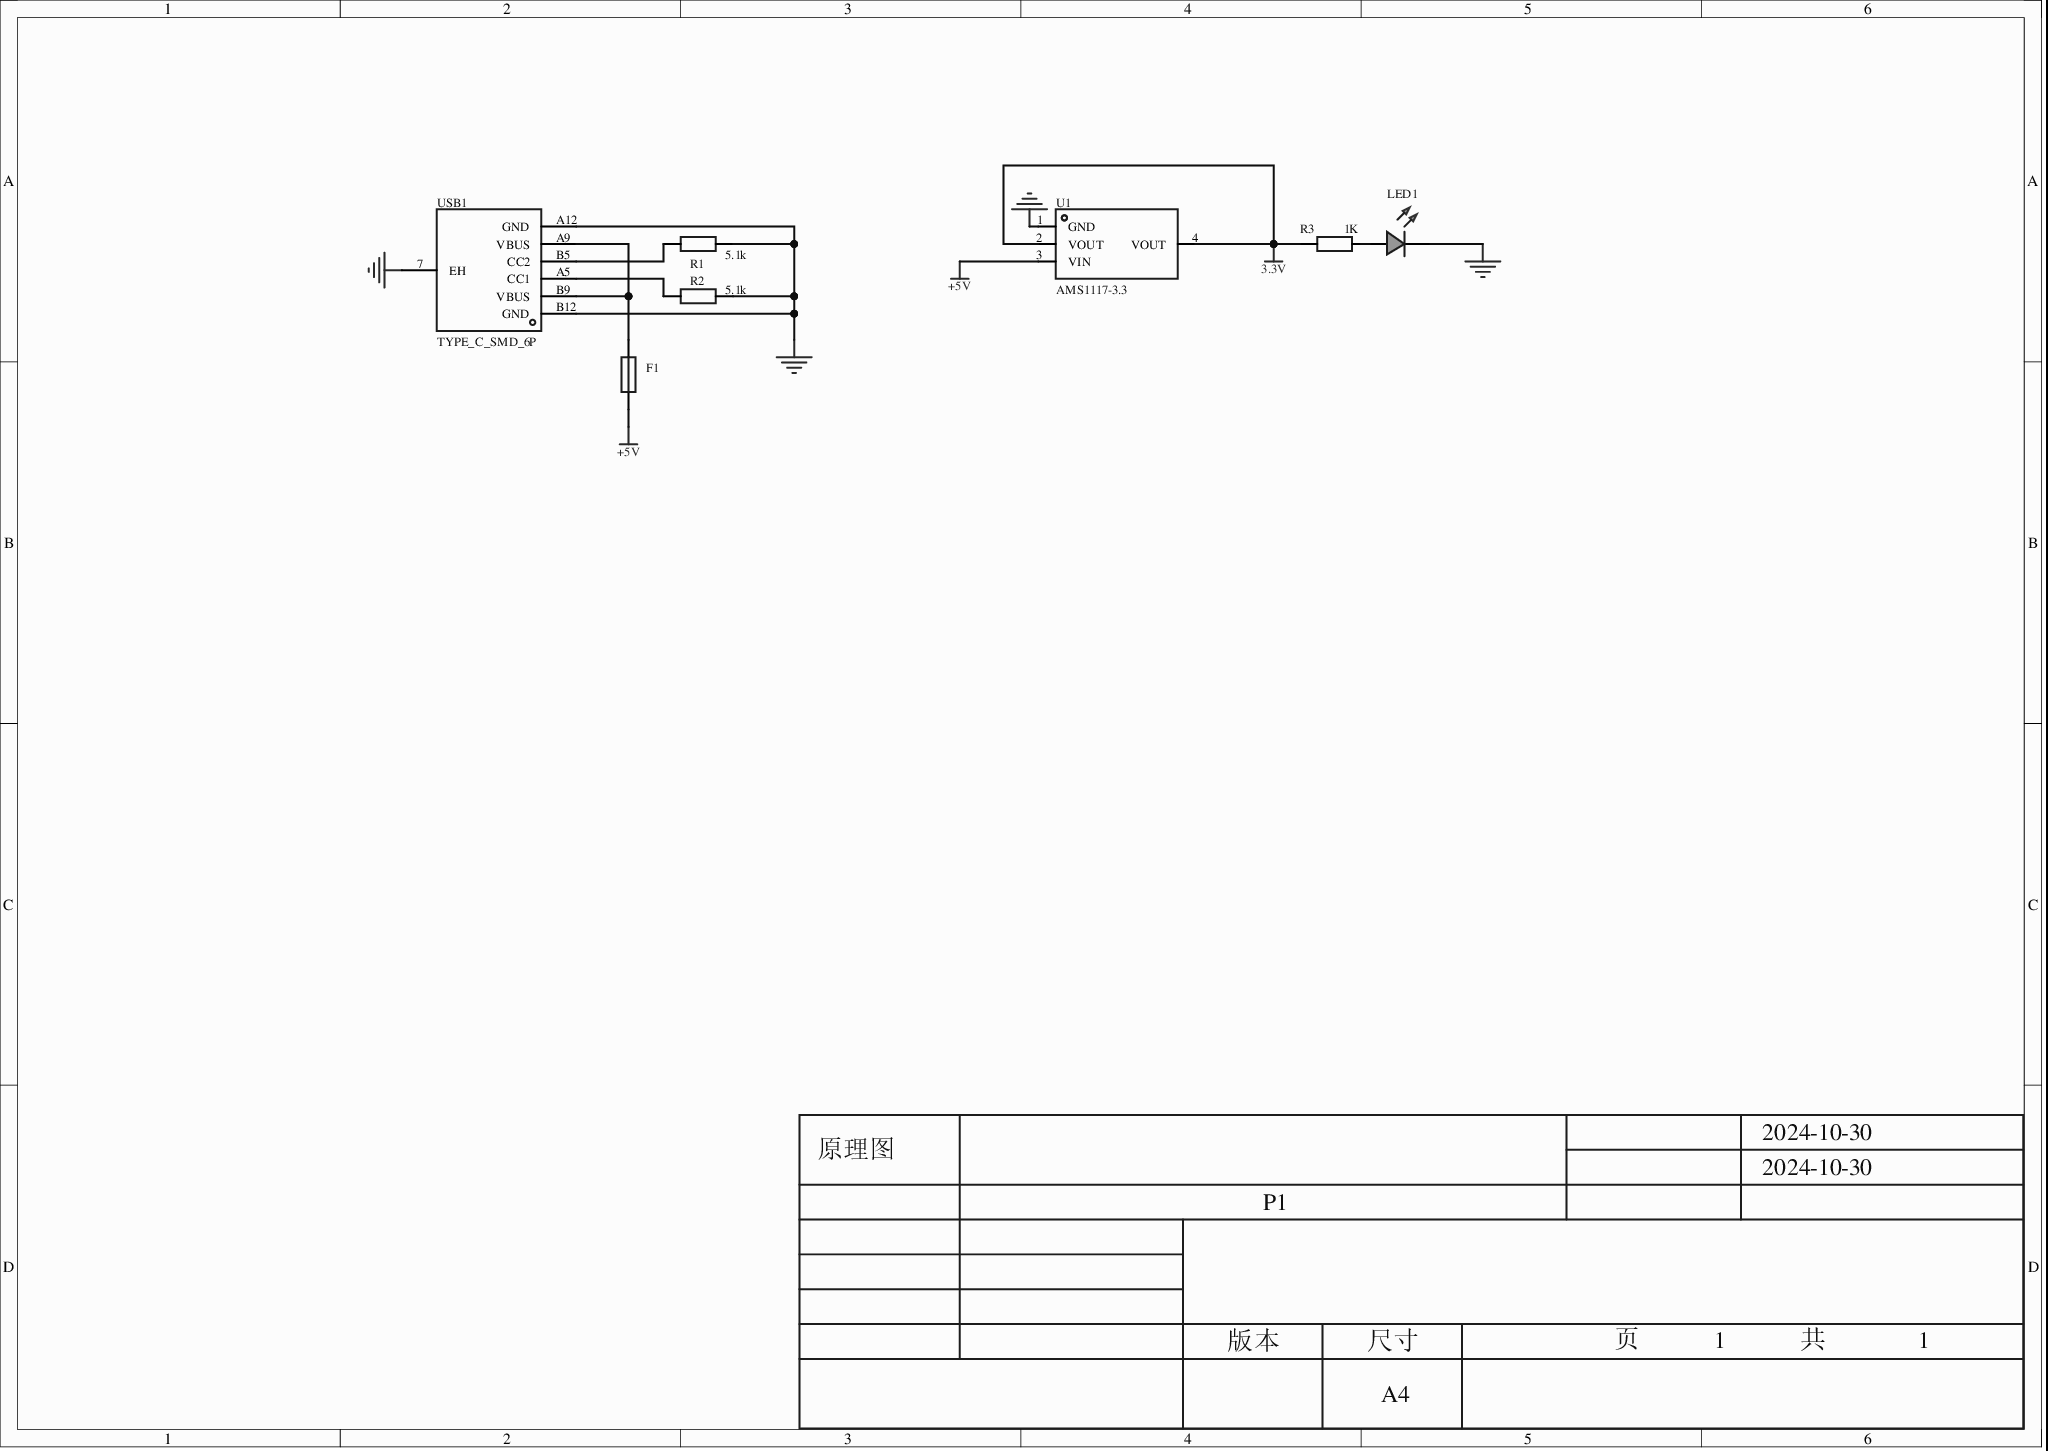
[diagram p0: MISC49884-3.schdoc]
# Altium project MISC49884-2.PrjPcb
1 sheet, 7 parts. Net scope: global (net labels, ports and power ports of the same name join across sheets).
Board file: MISC49884.pcbdoc

## Sheet MISC49884-3.schdoc
size 297 x 210 mm; Version: V1.0; @Project Name: MISC49884; @Page Count: 1; @Update Date: 2024-10-30; @Create Date: 2024-10-30; @Schematic Name: MISC49884; @Page No: 1

### Parts
F1  BSMD1206-200-6V  [F1206]  (value not drawn)
LED1  (no value)  [LED_0805]
R1  5.1k  [R0805]
R2  5.1k  [R0805]
R3  1K  [R0603]
U1  AMS1117-3.3  [SOT-223-3_L6.5-W3.4-P2.30-LS7.0-BR]
USB1  TYPE_C_SMD_6P  [TYPE-C-SMD_TYPE-C-6P]

### Nets
3.3V: R3.1 U1.2(VOUT) U1.4(VOUT)
+5V: F1.1 U1.3(VIN)
GND: LED1.1(C) R1.2 R2.2 U1.1(GND) USB1.7(EH) USB1.A12(GND) USB1.B12(GND)
NetF1_2: F1.2 USB1.A9(VBUS) USB1.B9(VBUS)
NetLED1_2: LED1.2(A) R3.2
NetR1_1: R1.1 USB1.B5(CC2)
NetR2_1: R2.1 USB1.A5(CC1)

### Notes on the sheet
- 2024-10-30
- 原理图
- P1
- 版本
- 尺寸
- A4
- 页
- 1
- 共

### Library data of the parts
F1 = BSMD1206-200-6V: 最大电压:6V;最大电流:100A;保持电流:2A;跳闸电流:3.5A;; Manufacturer: BHFUSE(佰宏); AddInBom: yes; ModelId: f1628daad26847a79b887277a2bc8541; ModelName: F1206_L3.2-W1.7-H0.6; ModelTransform: 125.984,66.929,0,0,0,0,0,0,0; Operating Voltage (Max): 6V; Current Rating (Max): 100A; Hold Current: 2A; Trip Current: 3.5A; Power Dissipation: 800mW; Resistance - Initial (Ri) (Min): 15mΩ; Resistance - Post Trip (R1) (Max): 80mΩ; Maximum Time to Trip: 1.5s; Symbol: BSMD1206-200-6V; Device: BSMD1206-200-6V; LCSC Part Name: 6V 2A 1206自恢复 1.5秒内动作; SupplierPart: C883134; ManufacturerPart: BSMD1206-200-6V; Supplier Footprint: 1206; JLCPCB Part Class: 扩展库; Datasheet: https://atta.szlcsc.com/upload/public/pdf/source/20220607/BE3D288249A8A8FEF08AA69BF9FC830E.pdf; Supplier: LCSC; ConvertToPcb: yes; FootprintName: F1206; Operating Temperature: -40℃~+85℃
LED1 = LED_0805-G: Symbol: LED_G; Convert to PCB: yes; 3D Model: 381ae4d721d6485eaad9d0ca067812b5; 3D Model Transform: 63.9,39.8,31.9,0,0,0,0,0,0; ModelName: LED-0805_G; Device: LED_0805-G; Add into BOM: yes; Supplier Footprint: 0805; FootprintName: LED_0805
R1 R2 = Res_0805: Symbol: 电阻; ConvertToPcb: yes; ModelId: 37a81e68749a4138bd2dfa6897b24b85; ModelName: R0805_L2.0-W1.3-H0.6; ModelTransform: 78.74,51.181,0,0,0,0,0,-0.0005,0; Value: 5.1k; Device: Res_0805; AddInBom: yes; Supplier Footprint: 0805; FootprintName: R0805
R3 = Res_0603: Symbol: 电阻; ConvertToPcb: yes; ModelId: fc143cca1e79419f9cd78b61e9279f08; ModelTransform: 31.8897,63.7794,0,90,0,0,0,0,0; Value: 1K; Device: Res_0603; AddInBom: yes; Supplier Footprint: 0603; FootprintName: R0603; ModelName: R0603
U1 = AMS1117-3.3_C6186: 输出类型:固定;最大输入电压:-;输出电压:3.3V;最大输出电流:1A;电源纹波抑制比(PSRR):72dB@(120Hz);输出极性:正极;; Manufacturer: AMS; AddInBom: yes; ModelId: 925194bf9823436183a3e0b978a8d076; ModelName: SOT-223-4P_L6.5-W3.5-H1.6-LS7.0-P2.30; ModelTransform: 279.89794,255.905,0,180,0,0,-3.9385,-0.0005,0; Output Type: 固定; Output Voltage: 3.3V; MAX Output Current: 1A; Dropout Voltage: 1.3V@(800mA); Output Polarity: 正极; Number of Outputs: 1; Symbol: AMS1117-3.3; Device: AMS1117-3.3_C6186; Supplier: LCSC; Manufacturer Part: AMS1117-3.3; Supplier Part: C6186; JLCPCB Part Class: 基础库; LCSC Part Name: 输出3.3V 1A; Supplier Footprint: SOT-223-3; Datasheet: https://atta.szlcsc.com/upload/public/pdf/source/20180727/C6186_7A095716F0823C02F1997A905E26C086.pdf; ConvertToPcb: yes; FootprintName: SOT-223-3_L6.5-W3.4-P2.30-LS7.0-BR; Maximum Input Voltage: -; Power Supply Rejection Ratio (PSRR): 72dB@(120Hz); standby current: -; Noise: -; Feature: -; Operating Temperature: -
USB1 = TYPE_C_SMD_6P: AddInBom: yes; ModelId: 3770c5585474407db939b2377e27177a; ModelName: TYPE-C-SMD_6P-L8.9-W6.8-H3.2-P1.00; ModelTransform: 351.9678,267.716,0,180,0,0,0,-45.766,-39.37; Symbol: TYPE_C_SMD_6P; Device: TYPE_C_SMD_6P; LCSC Part Name: TYPE_C_SMD_6P; SupplierPart: C9900003080; ManufacturerPart: TYPE_C_SMD_6P; Supplier Footprint: TYPE_C_USB_6P; JLCPCB Part Class: 扩展库; Supplier: LCSC; ConvertToPcb: yes; FootprintName: TYPE-C-SMD_TYPE-C-6P